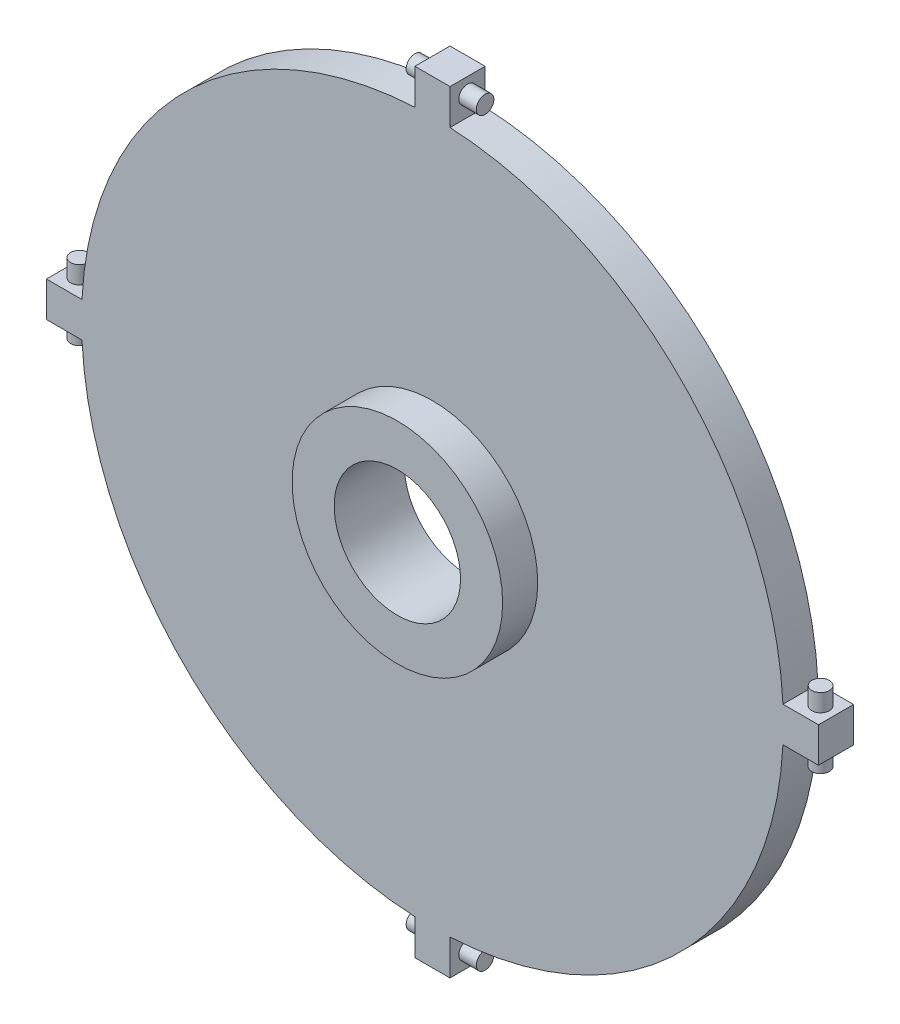
SolidWorks part; units mm, degrees
ref_plane "Front Plane" through (0, 0, 0) normal (0, 0, 1) x (1, 0, 0)
ref_plane "Top Plane" through (0, 0, 0) normal (0, 1, 0) x (1, 0, 0)
ref_plane "Right Plane" through (0, 0, 0) normal (1, 0, 0) x (0, 0, -1)
other "Configuration Table"
sketch "Sketch1" plane through (0, 0, 0) normal (0, 0, 1) x (1, 0, 0)
  circle A0 centre (0, 0) radius 50
  dimension "D1" = 100
extrude "Boss-Extrude1" add sketch "Sketch1" along normal blind 5
sketch "Sketch2" plane through (0, 0, 5) normal (0, 0, 1) x (1, 0, 0)
  circle A0 centre (0, 0) radius 15
  dimension "D1" = 30
extrude "Boss-Extrude2" add sketch "Sketch2" along normal blind 5
sketch "Sketch3" plane through (0, 0, 10) normal (0, 0, 1) x (1, 0, 0)
  circle A0 centre (0, 0) radius 9
  dimension "D1" = 18
extrude "Cut-Extrude1" cut sketch "Sketch3" against normal blind 15
ref_plane "Plane1" through (0, 55, 0) normal (0, 1, 0) x (1, 0, 0)
sketch "Sketch4" plane through (0, 55, 0) normal (0, 1, 0) x (1, 0, 0)
  line L0 (0, 0) -> (2.5, 0)
  line L1 (50, 0) -> (-50, 0) construction
  line L2 (9, 0) -> (-9, 0) construction
  line L3 (2.5, 0) -> (2.5, -5)
  line L4 (-15, -5) -> (15, -5) construction
  line L5 (2.5, -5) -> (-2.5, -5)
  line L6 (-2.5, -5) -> (-2.5, 0)
  line L7 (-2.5, 0) -> (0, 0)
  dimension "D1" = 2.5
  dimension "D2" = 2.5
extrude "Boss-Extrude3" add sketch "Sketch4" against normal up to surface (5.0625 mm away)
sketch "Sketch6" plane through (0, 0, 0) normal (1, 0, 0) x (0, 0, -1)
  line L0 (-5, 55) -> (0, 55) construction
  circle A0 centre (-2.5, 52.8) radius 1.25
  dimension "D1" = 2.5
  dimension "D2" = 2.2
extrude "Boss-Extrude4" add sketch "Sketch6" along normal mid plane 10
pattern_circular "CirPattern3" count 4 over 360 about axis through (0, 0, 0) along (0, 0, 1) of "Boss-Extrude3", "Boss-Extrude4"
